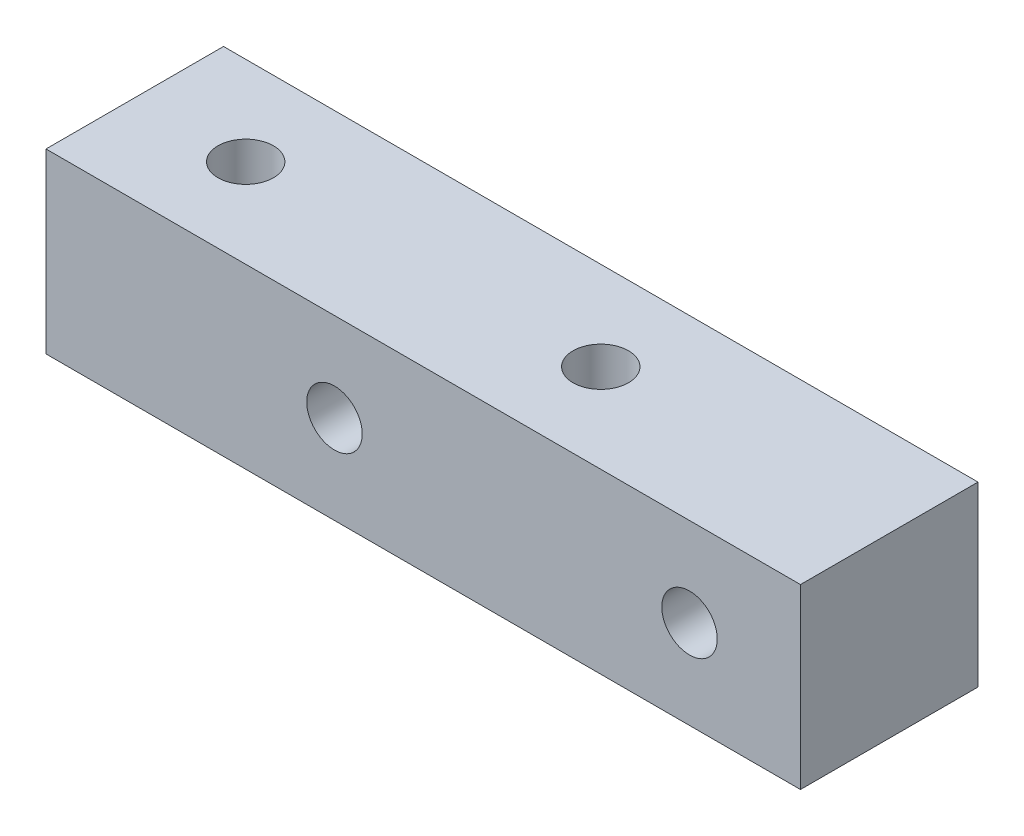
from build123d import *

# Parameters (mm, degrees)
SKETCH_1_W         = 34
SKETCH_1_H         = 8
EXTRUDE_1_DEPTH    = 8
HOLE_WIZARD_M3_1_D = 2.5
HOLE_WIZARD_M3_2_D = 2.5


with BuildPart() as part:
    # 草图1 → 凸台-拉伸1 (new body)
    with BuildSketch(Plane(origin=(0, 0, 0), x_dir=(1, 0, 0), z_dir=(0, 1, 0))):
        Rectangle(SKETCH_1_W, SKETCH_1_H)
    extrude(amount=EXTRUDE_1_DEPTH)

    # M3 螺纹孔1 (through all)
    with Locations(Plane(origin=(0, 8, 0), x_dir=(1, 0, 0), z_dir=(0, 1, 0))):
        with Locations((4, 0), (-12, 0)):
            Hole(HOLE_WIZARD_M3_1_D / 2)

    # M3 螺纹孔2 (through all)
    with Locations(Plane.XY.offset(4)):
        with Locations((12, 4), (-4, 4)):
            Hole(HOLE_WIZARD_M3_2_D / 2)


solid = part.part
